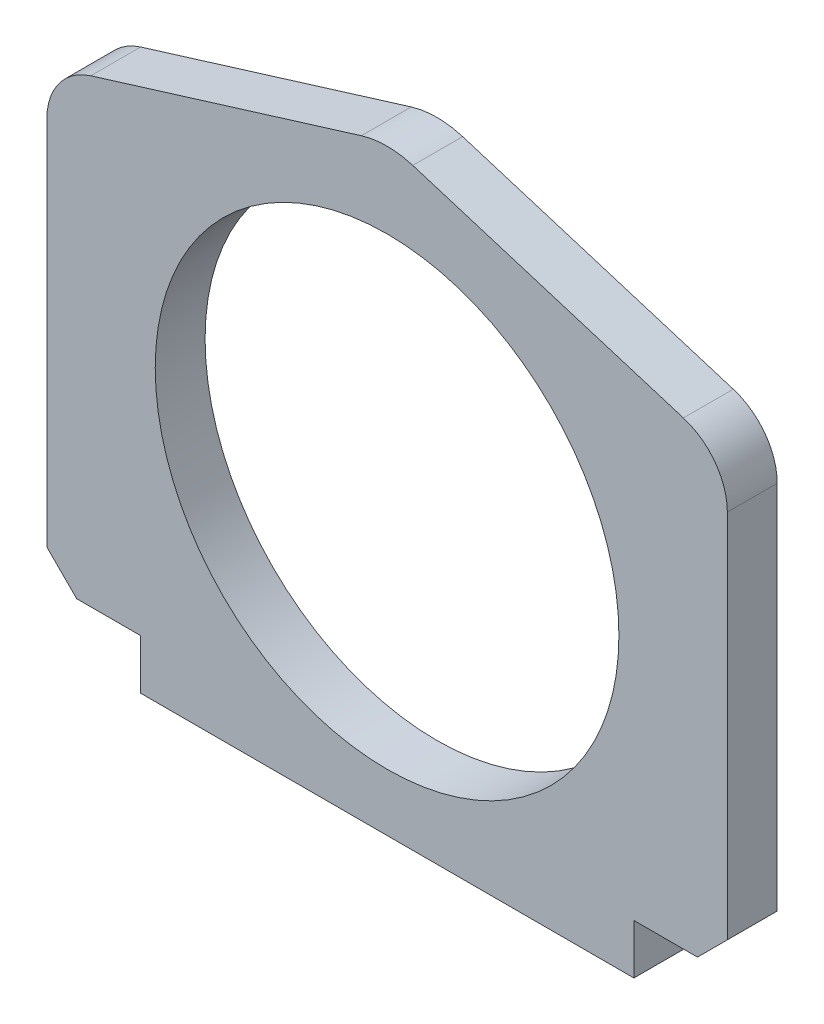
from build123d import *

# Parameters (mm, degrees)
SKETCH1_R           = 93
BOSS_EXTRUDE1_DEPTH = 20


with BuildPart() as part:
    # Sketch1 → Boss-Extrude1 (new body)
    with BuildSketch(Plane.XY):
        with BuildLine():
            Line((-99, 0), (99, 0))
            Line((99, 0), (99, 20))
            Line((99, 20), (124.5, 20))
            Line((124.5, 20), (136.5, 32))
            Line((136.5, 32), (136.5, 180.6))
            ThreePointArc((136.5, 180.6), (131.613179244, 195.447896171), (118.863198343, 204.491071767))
            Line((118.863198343, 204.491071767), (10.30847768, 237.947500473))
            ThreePointArc((10.30847768, 237.947500473), (0, 239.5), (-10.30847768, 237.947500473))
            Line((-10.30847768, 237.947500473), (-118.863198343, 204.491071767))
            ThreePointArc((-118.863198343, 204.491071767), (-131.613179244, 195.447896171), (-136.5, 180.6))
            Line((-136.5, 180.6), (-136.5, 32))
            Line((-136.5, 32), (-124.5, 20))
            Line((-124.5, 20), (-99, 20))
            Line((-99, 20), (-99, 0))
        make_face()
        with Locations((0, 116)):
            Circle(SKETCH1_R, mode=Mode.SUBTRACT)
    extrude(amount=BOSS_EXTRUDE1_DEPTH)


solid = part.part
